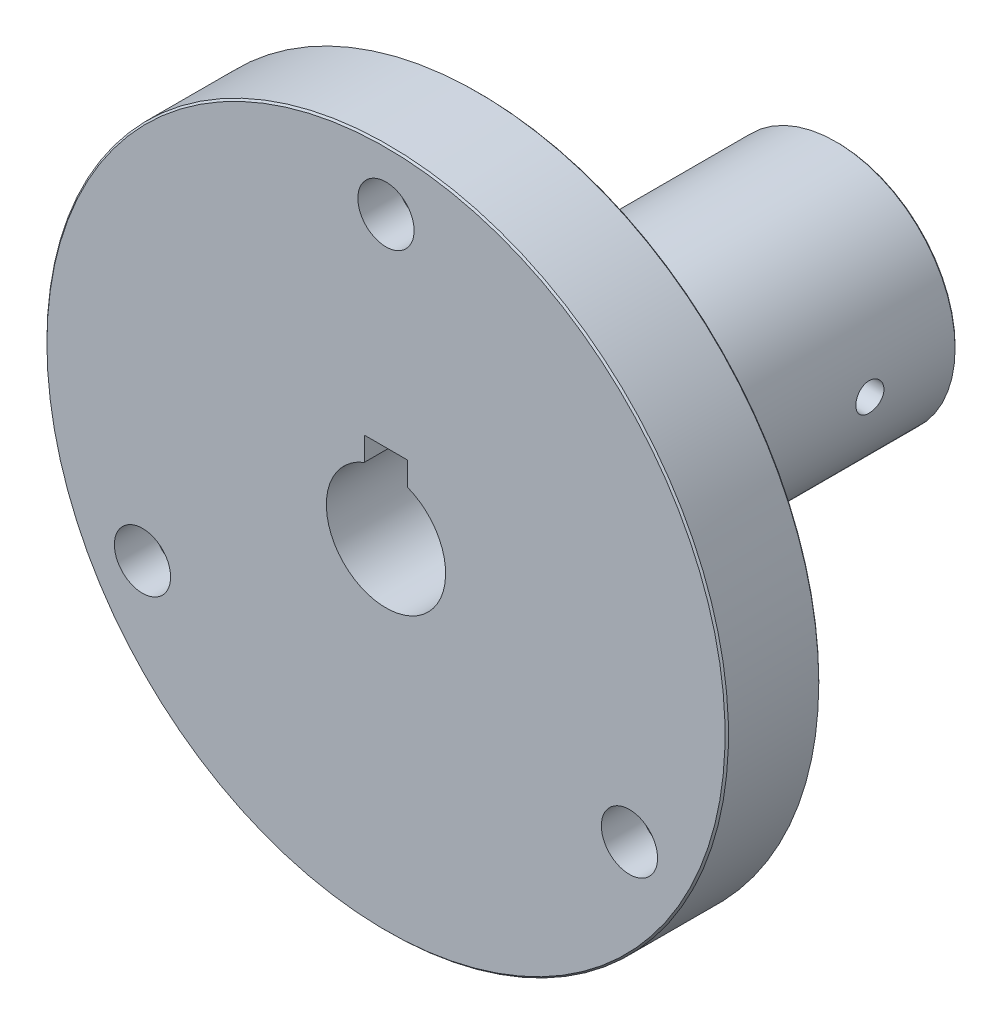
SolidWorks part; units mm, degrees
material "6061"
ref_plane "前视基准面" through (0, 0, 0) normal (0, 0, 1) x (1, 0, 0)
ref_plane "上视基准面" through (0, 0, 0) normal (0, 1, 0) x (1, 0, 0)
ref_plane "右视基准面" through (0, 0, 0) normal (1, 0, 0) x (0, 0, -1)
sketch "草图1" plane through (0, 0, 0) normal (0, 0, 1) x (1, 0, 0)
  circle A0 centre (0, 0) radius 14
  dimension "D1" = 28
extrude "凸台-拉伸1" add sketch "草图1" along normal blind 42
sketch "草图2" plane through (0, 0, 42) normal (0, 0, 1) x (1, 0, 0)
  circle A0 centre (0, 0) radius 40
  dimension "D1" = 80
extrude "凸台-拉伸2" add sketch "草图2" along normal blind 11
sketch "草图3" plane through (0, 0, 0) normal (0, 0, -1) x (-1, 0, 0)
  circle A0 centre (0, 0) radius 7
  dimension "D1" = 14
extrude "切除-拉伸1" cut sketch "草图3" against normal through all
hole_wizard "M6 六角凹头螺钉的柱形沉头孔1" positions "草图5" profile "草图4" counterbore size "M6" standard "ISO" end condition through all
sketch "草图5" plane through (0, 0, 42) normal (0, 0, -1) x (-1, 0, 0)
  point P0 (0, 33)
  dimension "D1" = 33
sketch "草图4" plane through (0, 33, 42) normal (1, 0, 0) x (0, 1, 0)
  line L0 (0, 0) -> (0, 11)
  line L1 (0, 11) -> (3.3, 11)
  line L3 (3.3, 11) -> (3.3, 6.4)
  line L4 (3.3, 6.4) -> (5.5, 6.4)
  line L5 (5.5, 6.4) -> (5.5, 0)
  line L7 (5.5, 0) -> (0, 0)
  line L11 (0, -6.35) -> (0, 107.95) construction
  dimension "通孔孔直径" = 6.6
  dimension "通孔孔深度" = 11
  dimension "柱形沉头孔直径" = 11
  dimension "柱形沉头孔深度" = 6.4
pattern_circular "阵列(圆周)1" count 3 over 360 about axis through (0, 0, 0) along (0, 0, 1) of "M6 六角凹头螺钉的柱形沉头孔1"
ref_plane "基准面1" through (0, -12, 0) normal (0, 1, 0) x (1, 0, 0)
sketch "草图9" plane through (0, -12, 0) normal (0, 1, 0) x (1, 0, 0)
  line L0 (14, 0) -> (-14, 0) construction
  line L1 (-15, -36) -> (15, -36)
  line L2 (-15, -36) -> (-15, -14)
  line L3 (-15, -14) -> (15, -14)
  line L4 (15, -36) -> (15, -14)
  line L5 (-15, -36) -> (15, -14) construction
  line L6 (-15, -14) -> (15, -36) construction
  point P0 (0, -25)
  dimension "D1" = 25
  dimension "D2" = 22
  dimension "D3" = 30
extrude "切除-拉伸3" cut sketch "草图9" against normal through all
hole_wizard "M4 螺纹孔2" positions "草图11" profile "草图10" tap size "M4" standard "GB"
sketch "草图11" plane through (0, -12, 0) normal (0, -1, 0) x (-1, 0, 0)
  line L0 (7.2111, -36) -> (-7.2111, -36) construction
  line L1 (-7.2111, -14) -> (7.2111, -14) construction
  point P0 (0, -30)
  point P2 (0, -22)
  dimension "D1" = 6
  dimension "D2" = 8
sketch "草图10" plane through (0, -12, 30) normal (1, 0, 0) x (0, 0, -1)
  line L0 (0, 0) -> (0, 12.4914)
  line L1 (0, 12.4914) -> (1.65, 11.5)
  line L2 (1.65, 11.5) -> (1.65, 0)
  line L5 (1.65, 0) -> (0, 0)
  line L10 (0, 12.4914) -> (-1.65, 11.5) construction
  line L11 (0, -6.35) -> (0, 107.95) construction
  dimension "螺纹孔钻头直径" = 3.3
  dimension "螺纹孔钻头深度" = 11.5
  dimension "导头角度" = 118
cosmetic thread "孔螺蚊线3" parameters "D1"=5.1972, "D2"=4
cosmetic thread "孔螺蚊线4" parameters "D1"=5.1972, "D2"=4
sketch "草图12" plane through (0, 0, 0) normal (0, 0, -1) x (-1, 0, 0)
  line L1 (-2.55, 4.7) -> (2.55, 4.7)
  line L2 (-2.55, 4.7) -> (-2.55, 9.3)
  line L3 (-2.55, 9.3) -> (2.55, 9.3)
  line L4 (2.55, 4.7) -> (2.55, 9.3)
  line L5 (-2.55, 4.7) -> (2.55, 9.3) construction
  line L6 (-2.55, 9.3) -> (2.55, 4.7) construction
  circle A0 centre (0, 0) radius 7 construction
  point P0 (0, 7)
  dimension "D1" = 9.3
  dimension "D2" = 5.1
extrude "切除-拉伸4" cut sketch "草图12" against normal through all
chamfer "倒角1" distance 0.2 angle 45 3 edges at (14, 0, 0) (40, 0, 42) (40, 0, 53)
fillet "圆角1" radius 1 1 edges at (14, 0, 42)
ref_plane "基准面2" through (15, 0, 0) normal (1, 0, 0) x (0, 0, -1)
hole_wizard "M4 螺纹孔3" positions "草图14" profile "草图13" tap size "M4" standard "GB" end condition through all
sketch "草图14" plane through (15, 0, 0) normal (1, 0, 0) x (0, 0, -1)
  line L0 (-0.2, 14) -> (-0.2, -14) construction
  point P0 (-10.2, 0)
  point P2 (-25.2, 0)
  dimension "D1" = 10
  dimension "D2" = 15
sketch "草图13" plane through (15, 0, 10.2) normal (0, 1, 0) x (0, 0, -1)
  line L0 (0, 0) -> (0, 55)
  line L1 (0, 55) -> (1.65, 55)
  line L2 (1.65, 55) -> (1.65, 0)
  line L5 (1.65, 0) -> (0, 0)
  line L11 (0, -6.35) -> (0, 107.95) construction
  dimension "通孔螺纹孔钻头直径" = 3.3
  dimension "通孔螺纹孔钻头深度" = 55
cosmetic thread "孔螺蚊线5" parameters "D2"=4
cosmetic thread "孔螺蚊线6" parameters "D2"=4
